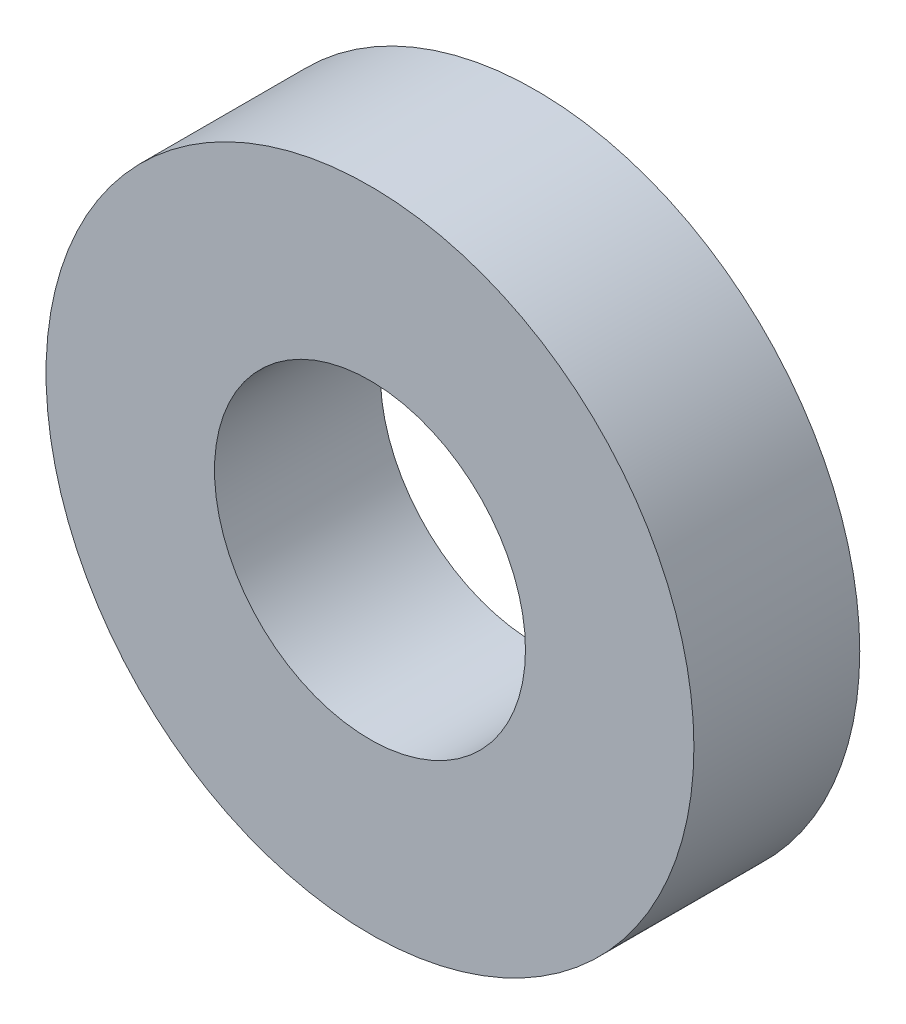
SolidWorks part; units mm, degrees
ref_plane "前视基准面" through (0, 0, 0) normal (0, 0, 1) x (1, 0, 0)
ref_plane "上视基准面" through (0, 0, 0) normal (0, 1, 0) x (1, 0, 0)
ref_plane "右视基准面" through (0, 0, 0) normal (1, 0, 0) x (0, 0, -1)
other "Configuration Table"
sketch "草图1" plane through (0, 0, 0) normal (0, 0, 1) x (1, 0, 0)
  circle A0 centre (0, 0) radius 62.5
  circle A1 centre (0, 0) radius 30
  point P0 (0, 0)
  dimension "D1" = 60
  dimension "D2" = 125
extrude "凸台-拉伸1" add sketch "草图1" against normal mid plane 32
